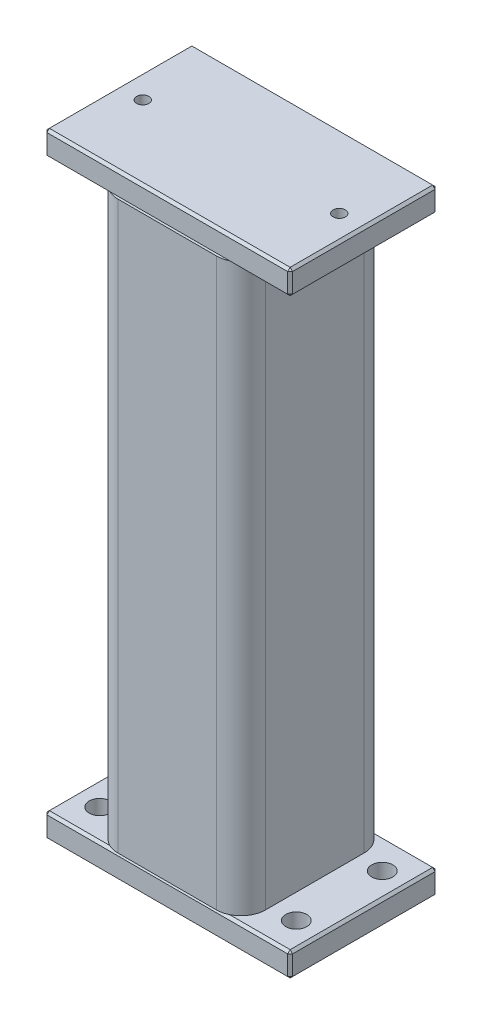
from build123d import *

# Parameters (mm, degrees)
MEMBER_1_DEPTH                   = 230.5
SKETCH_2_W                       = 100
SKETCH_2_H                       = 60
EXTRUDE_1_DEPTH                  = 10
SKETCH_3_W                       = 100
SKETCH_3_H                       = 60
EXTRUDE_2_DEPTH                  = 10
CHAMFER_1_SIZE                   = 1
CHAMFER_2_SIZE                   = 1
HOLE_WIZARD_8_6_8_6_1_AT_2_COUNT = 2
HOLE_WIZARD_8_6_8_6_1_AT_2_PITCH = 35
HOLE_WIZARD_8_6_8_6_1_AT_3_COUNT = 2
HOLE_WIZARD_8_6_8_6_1_AT_3_PITCH = 80
HOLE_WIZARD_8_6_8_6_1_AT_4_COUNT = 2
HOLE_WIZARD_8_6_8_6_1_AT_4_PITCH = 87.321245983
HOLE_WIZARD_M6_1_AT_2_COUNT      = 2
HOLE_WIZARD_M6_1_AT_2_PITCH      = 80


with BuildPart() as part:
    # Sketch11 → Member 1 (new body)
    with BuildSketch(Plane(origin=(0, 0, 0), x_dir=(1, 0, 0), z_dir=(0, 1, 0))):
        with BuildLine():
            Line((-20, -30), (20, -30))
            ThreePointArc((20, -30), (27.071067812, -27.071067812), (30, -20))
            Line((30, -20), (30, 20))
            ThreePointArc((30, 20), (27.071067812, 27.071067812), (20, 30))
            Line((20, 30), (-20, 30))
            ThreePointArc((-20, 30), (-27.071067812, 27.071067812), (-30, 20))
            Line((-30, 20), (-30, -20))
            ThreePointArc((-30, -20), (-27.071067812, -27.071067812), (-20, -30))
        make_face()
        with BuildLine():
            Line((-20, -25), (20, -25))
            ThreePointArc((20, -25), (23.535533906, -23.535533906), (25, -20))
            Line((25, -20), (25, 20))
            ThreePointArc((25, 20), (23.535533906, 23.535533906), (20, 25))
            Line((20, 25), (-20, 25))
            ThreePointArc((-20, 25), (-23.535533906, 23.535533906), (-25, 20))
            Line((-25, 20), (-25, -20))
            ThreePointArc((-25, -20), (-23.535533906, -23.535533906), (-20, -25))
        make_face(mode=Mode.SUBTRACT)
    extrude(amount=MEMBER_1_DEPTH)


with BuildPart() as body_2:
    # 草图2 → 凸台-拉伸1 (new body)
    with BuildSketch(Plane(origin=(0, 230.5, 0), x_dir=(1, 0, 0), z_dir=(0, 1, 0))):
        Rectangle(SKETCH_2_W, SKETCH_2_H)
    extrude(amount=EXTRUDE_1_DEPTH)

    # 倒角1
    chamfer_1_edges = [body_2.edges().sort_by_distance(p)[0] for p in [
        (-50, 240.5, 0),
        (0, 240.5, 30),
        (50, 240.5, 0),
        (0, 230.5, 30),
        (-50, 230.5, 0),
        (0, 230.5, -30),
        (50, 230.5, 0),
        (0, 240.5, -30),
        (50, 235.5, 30),
        (-50, 235.5, 30),
        (-50, 235.5, -30),
        (50, 235.5, -30),
    ]]
    chamfer(chamfer_1_edges, length=CHAMFER_1_SIZE)

    # 草图11 → M6 螺纹孔1 (revolve, cut)
    with BuildSketch(Plane(origin=(-40, 240.5, 0), x_dir=(0, 0, 1), z_dir=(1, 0, 0))):
        Polygon((0, 0), (0, 18.502151548), (2.5, 17), (2.5, 0), align=None)
    hole_wizard_m6_1 = revolve(axis=Axis((-40, 246.85, 0), (0, -1, 0)), mode=Mode.SUBTRACT)

    # M6 螺纹孔1 at 2: M6 螺纹孔1 ×2
    with Locations(*[(i * HOLE_WIZARD_M6_1_AT_2_PITCH, 0, 0) for i in range(1, HOLE_WIZARD_M6_1_AT_2_COUNT)]):
        add(hole_wizard_m6_1, mode=Mode.SUBTRACT)


with BuildPart() as body_3:
    # 草图3 → 凸台-拉伸2 (new body)
    with BuildSketch(Plane.XZ):
        Rectangle(SKETCH_3_W, SKETCH_3_H)
    extrude(amount=EXTRUDE_2_DEPTH)

    # 倒角2
    chamfer_2_edges = [body_3.edges().sort_by_distance(p)[0] for p in [
        (-50, -10, 0),
        (0, -10, -30),
        (50, -10, 0),
        (0, 0, -30),
        (-50, 0, 0),
        (0, 0, 30),
        (50, 0, 0),
        (0, -10, 30),
        (50, -5, -30),
        (-50, -5, -30),
        (-50, -5, 30),
        (50, -5, 30),
    ]]
    chamfer(chamfer_2_edges, length=CHAMFER_2_SIZE)

    # 草图4 → Ø8.6 (8.6) 直径孔1 (revolve, cut)
    with BuildSketch(Plane(origin=(40, 0, -17.5), x_dir=(0, 0, 1), z_dir=(1, 0, 0))):
        Polygon((0, 0), (0, 18.092606158), (4.3, 15.61), (4.3, 0), align=None)
    hole_wizard_8_6_8_6_1 = revolve(axis=Axis((40, 6.35, -17.5), (0, -1, 0)), mode=Mode.SUBTRACT)

    # Ø8.6 (8.6) 直径孔1 at 2: Ø8.6 (8.6) 直径孔1 ×2
    with Locations(*[(0, 0, i * HOLE_WIZARD_8_6_8_6_1_AT_2_PITCH) for i in range(1, HOLE_WIZARD_8_6_8_6_1_AT_2_COUNT)]):
        add(hole_wizard_8_6_8_6_1, mode=Mode.SUBTRACT)

    # Ø8.6 (8.6) 直径孔1 at 3: Ø8.6 (8.6) 直径孔1 ×2
    with Locations(*[(-i * HOLE_WIZARD_8_6_8_6_1_AT_3_PITCH, 0, 0) for i in range(1, HOLE_WIZARD_8_6_8_6_1_AT_3_COUNT)]):
        add(hole_wizard_8_6_8_6_1, mode=Mode.SUBTRACT)

    # Ø8.6 (8.6) 直径孔1 at 4: Ø8.6 (8.6) 直径孔1 ×2
    with Locations(*[Vector(-0.9161573349021891, 0, 0.4008188340197079) * (i * HOLE_WIZARD_8_6_8_6_1_AT_4_PITCH) for i in range(1, HOLE_WIZARD_8_6_8_6_1_AT_4_COUNT)]):
        add(hole_wizard_8_6_8_6_1, mode=Mode.SUBTRACT)


solid = Compound([part.part, body_2.part, body_3.part])
